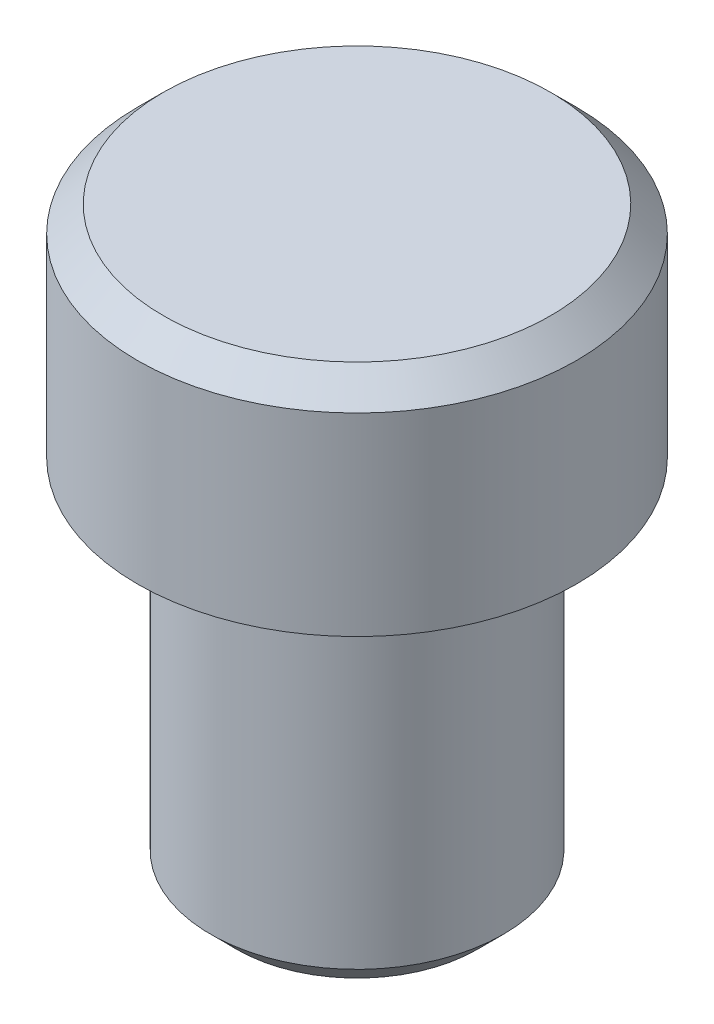
SolidWorks part; units mm, degrees
material "S45C"
ref_plane "Front" through (0, 0, 0) normal (0, 0, 1) x (1, 0, 0)
ref_plane "Top" through (0, 0, 0) normal (0, 1, 0) x (1, 0, 0)
ref_plane "Right" through (0, 0, 0) normal (1, 0, 0) x (0, 0, -1)
sketch "Sketch1" plane through (0, 0, 0) normal (0, 0, 1) x (1, 0, 0)
  line L0 (0, 0) -> (5.2929, 0)
  line L1 (5.2929, 0) -> (6, -0.7071)
  line L2 (6, -0.7071) -> (6, -6)
  line L3 (6, -6) -> (5, -6)
  line L4 (5, -6) -> (4.5, -5.5)
  line L5 (4.5, -5.5) -> (4, -5.5)
  line L6 (3.5, -6) -> (3.5, -6.5)
  line L7 (3.5, -6.5) -> (4, -7)
  line L8 (4, -7) -> (4, -15.2929)
  line L9 (4, -15.2929) -> (3.2929, -16)
  line L10 (3.2929, -16) -> (0, -16)
  line L11 (0, 42.1705) -> (0, -9.5264) construction
  line L12 (0, 0) -> (0, -16)
  arc A0 (4, -5.5) -> (3.5, -6) centre (4, -6) ccw
  dimension "D6" = 0.5
  dimension "D3" = 45
  dimension "D4" = 45
  dimension "D5" = 45
  dimension "H" = 6
  dimension "D8" = 45
  dimension "D_" = 12
  dimension "d" = 8
  dimension "L" = 16
revolve "Boss-Revolve" add sketch "Sketch1" angle 360 about L11
